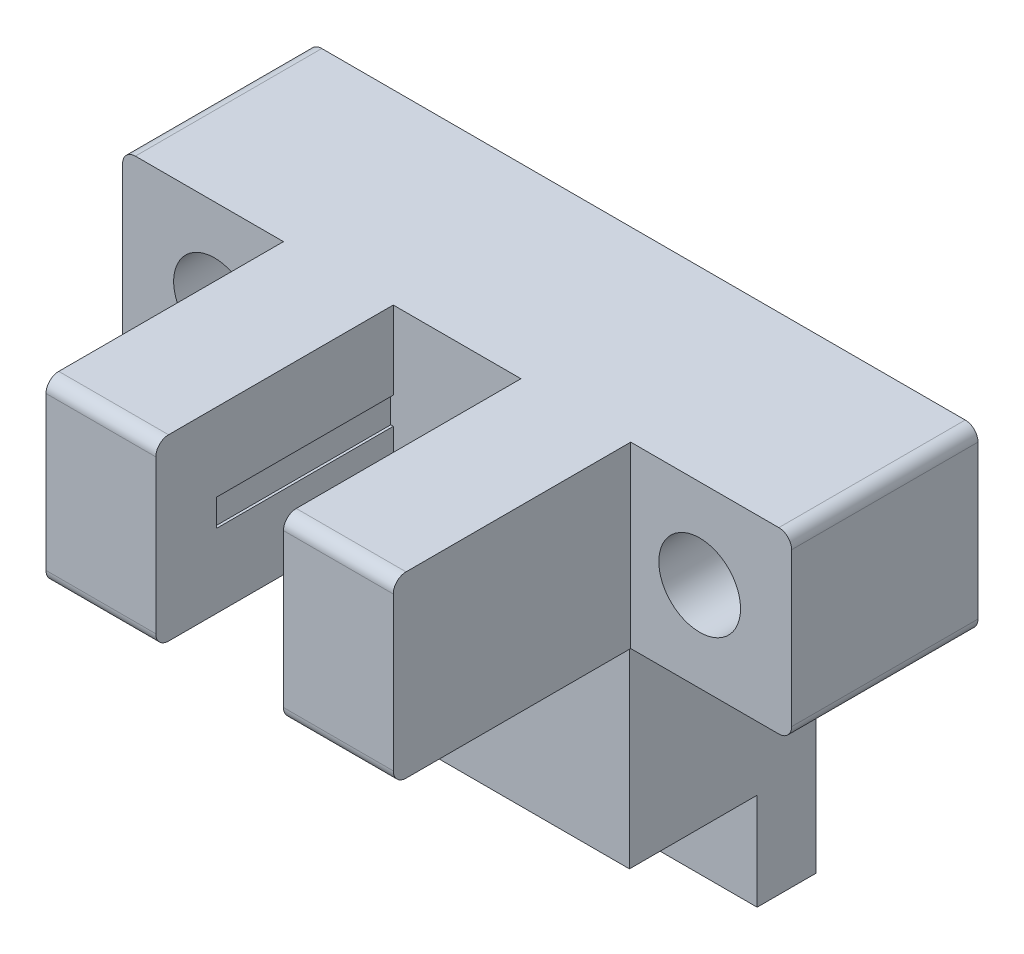
from build123d import *

# Parameters (mm, degrees)
SKETCH_1_W          = 26.2
SKETCH_1_H          = 18.3
EXTRUDE_1_DEPTH     = 7.3
SKETCH_2_W          = 6.35
SKETCH_2_H          = 11.3
CUT_EXTRUDE_1_DEPTH = 18.567654937
SKETCH_3_W          = 4.3
SKETCH_3_H          = 7
EXTRUDE_2_DEPTH     = 9.3
SKETCH_4_W          = 13.5
SKETCH_4_H          = 3.8
CUT_EXTRUDE_2_DEPTH = 5
SKETCH_5_R          = 1.6
CUT_EXTRUDE_3_DEPTH = 19.488442336
SKETCH_6_W          = 6.920128801
SKETCH_6_H          = 1.058382597
CUT_EXTRUDE_4_DEPTH = 0.1
FILLET_1_R          = 0.5
FILLET_2_R          = 0.5


with BuildPart() as part:
    # 草图1 → 凸台-拉伸1 (new body)
    with BuildSketch(Plane.XY):
        Rectangle(SKETCH_1_W, SKETCH_1_H)
    extrude(amount=EXTRUDE_1_DEPTH)

    # 草图2 → 切除-拉伸1 (cut, through all)
    with BuildSketch(Plane.XY.offset(7.3)):
        with Locations((-9.925, -3.5)):
            Rectangle(SKETCH_2_W, SKETCH_2_H)
        with Locations((9.925, -3.5)):
            Rectangle(SKETCH_2_W, SKETCH_2_H)
    extrude(amount=-CUT_EXTRUDE_1_DEPTH, mode=Mode.SUBTRACT)

    # 草图3 → 凸台-拉伸2 (add)
    with BuildSketch(Plane.XY.offset(7.3)):
        with Locations((-4.65, 5.65)):
            Rectangle(SKETCH_3_W, SKETCH_3_H)
        with Locations((4.65, 5.65)):
            Rectangle(SKETCH_3_W, SKETCH_3_H)
    extrude(amount=EXTRUDE_2_DEPTH)

    # 草图4 → 切除-拉伸2 (cut)
    with BuildSketch(Plane.XY.offset(7.3)):
        with Locations((0, -7.25)):
            Rectangle(SKETCH_4_W, SKETCH_4_H)
    extrude(amount=-CUT_EXTRUDE_2_DEPTH, mode=Mode.SUBTRACT)

    # 草图5 → 切除-拉伸3 (cut, through all)
    with BuildSketch(Plane.XY.offset(7.3)):
        with Locations((-9.5, 5.65)):
            Circle(SKETCH_5_R)
        with Locations((9.5, 5.65)):
            Circle(SKETCH_5_R)
    extrude(amount=-CUT_EXTRUDE_3_DEPTH, mode=Mode.SUBTRACT)

    # 草图6 → 切除-拉伸4 (cut)
    with BuildSketch(Plane(origin=(-2.5, 0, 0), x_dir=(0, 0, -1), z_dir=(1, 0, 0))):
        with Locations((-10.760064401, 5.564886087)):
            Rectangle(SKETCH_6_W, SKETCH_6_H)
    cut_extrude_4 = extrude(amount=-CUT_EXTRUDE_4_DEPTH, mode=Mode.SUBTRACT)

    # 圆角1
    fillet_1_edges = [part.edges().sort_by_distance(p)[0] for p in [
        (13.1, 2.15, 3.65),
        (13.1, 9.15, 3.65),
        (-13.1, 2.15, 3.65),
        (-13.1, 9.15, 3.65),
    ]]
    fillet(fillet_1_edges, radius=FILLET_1_R)

    # 镜向1: 切除-拉伸4 across plane
    add(cut_extrude_4.mirror(Plane(origin=(0, 0, 0), x_dir=(0, 0, 1), z_dir=(1, 0, 0))), mode=Mode.SUBTRACT)

    # 圆角2
    fillet_2_edges = [part.edges().sort_by_distance(p)[0] for p in [
        (4.65, 2.15, 16.6),
        (4.65, 9.15, 16.6),
        (-4.65, 9.15, 16.6),
        (-4.65, 2.15, 16.6),
    ]]
    fillet(fillet_2_edges, radius=FILLET_2_R)


solid = part.part
